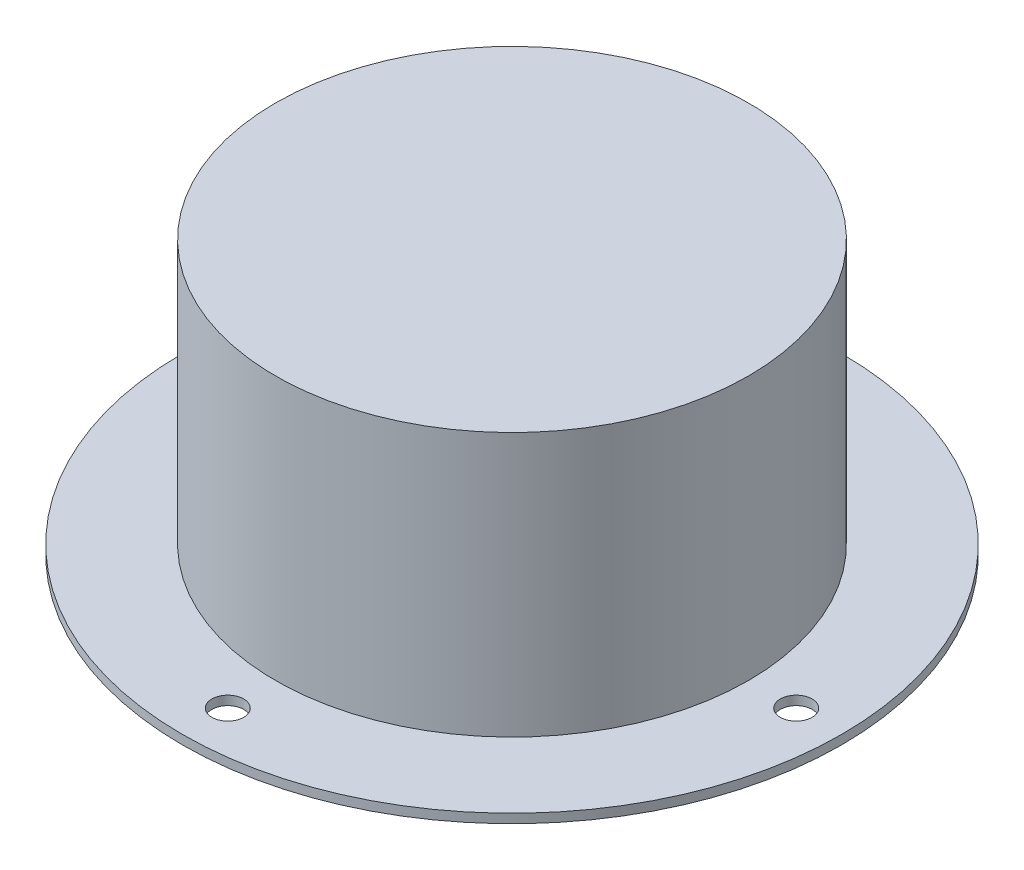
from build123d import *

# Parameters (mm, degrees)
SKETCH2_R          = 3.5
CUT_EXTRUDE1_DEPTH = 118.798556867
CIRPATTERN1_COUNT  = 4


with BuildPart() as part:
    # Sketch1 → Revolve1 (revolve)
    with BuildSketch(Plane.XY):
        Polygon((-50, 0), (-72.5, 0), (-72.5, 2), (-52, 2), (-52, 60), (0, 60), (0, 58), (-50, 58), align=None)
    revolve(axis=Axis((0, 60, 0), (0, -1, 0)))

    # Sketch2 → Cut-Extrude1 (cut, through all)
    with BuildSketch(Plane(origin=(0, 2, 0), x_dir=(1, 0, 0), z_dir=(0, 1, 0))):
        with Locations(Location((0, 62.5, 0), (0, 0, 180))):
            Circle(SKETCH2_R)
    cut_extrude1 = extrude(amount=-CUT_EXTRUDE1_DEPTH, mode=Mode.SUBTRACT)

    # CirPattern1: Cut-Extrude1 ×4 about axis
    cirpattern1_axis = Axis((0, 0, 0), (0, 1, 0))
    for i in range(1, CIRPATTERN1_COUNT):
        add(cut_extrude1.rotate(cirpattern1_axis, i * 360 / CIRPATTERN1_COUNT), mode=Mode.SUBTRACT)


solid = part.part
